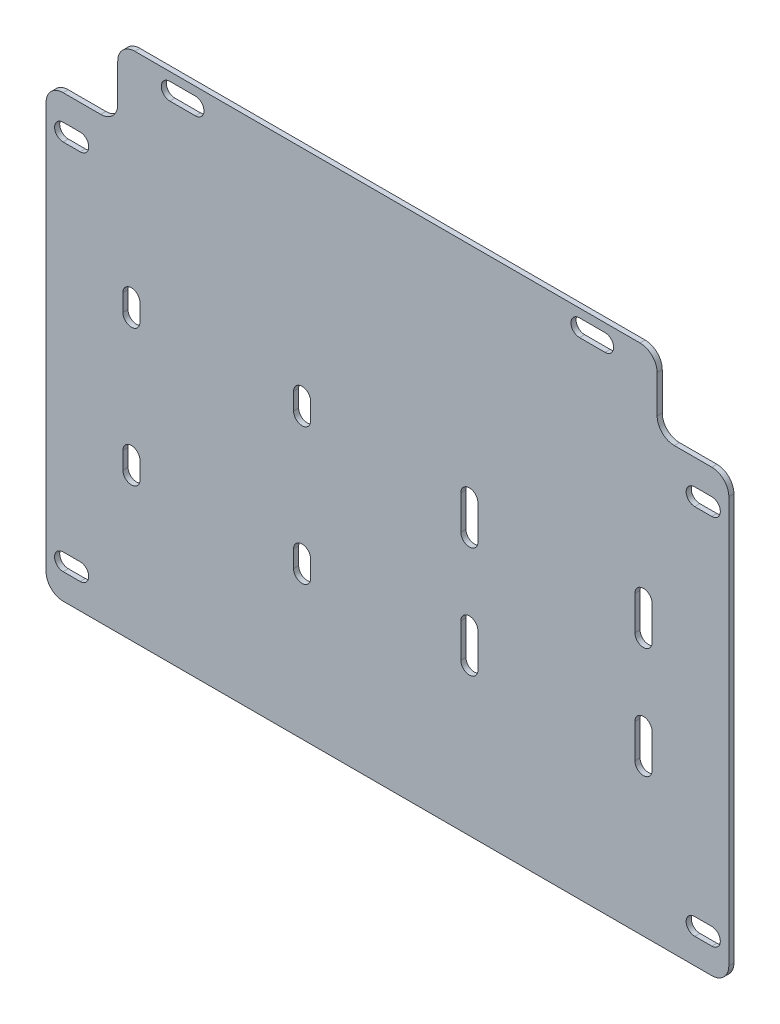
SolidWorks part; units mm, degrees
ref_plane "Front Plane" through (0, 0, 0) normal (0, 0, 1) x (1, 0, 0)
ref_plane "Top Plane" through (0, 0, 0) normal (0, 1, 0) x (1, 0, 0)
ref_plane "Right Plane" through (0, 0, 0) normal (1, 0, 0) x (0, 0, -1)
other "Configuration Table"
sketch "Sketch1" plane through (0, 0, 0) normal (0, 0, 1) x (1, 0, 0)
  line L0 (248, -128.5) -> (248, -148.5) construction
  line L1 (0, 0) -> (400, 0)
  line L2 (0, 0) -> (0, -342)
  line L3 (0, -342) -> (400, -342)
  line L4 (400, 0) -> (400, -342)
  line L5 (253, -128.5) -> (253, -148.5)
  line L6 (243, -128.5) -> (243, -148.5)
  line L7 (200, 0) -> (200, -342) construction
  line L8 (0, -171) -> (400, -171) construction
  line L9 (350, -128.5) -> (350, -148.5) construction
  line L10 (345, -128.5) -> (345, -148.5)
  line L11 (355, -128.5) -> (355, -148.5)
  line L12 (350, -213.5) -> (350, -193.5) construction
  line L13 (345, -213.5) -> (345, -193.5)
  line L14 (355, -213.5) -> (355, -193.5)
  line L15 (248, -213.5) -> (248, -193.5) construction
  line L16 (253, -213.5) -> (253, -193.5)
  line L17 (243, -213.5) -> (243, -193.5)
  line L18 (72.5, -10) -> (87.5, -10) construction
  line L19 (72.5, -5) -> (87.5, -5)
  line L20 (72.5, -15) -> (87.5, -15)
  line L21 (327.5, -10) -> (312.5, -10) construction
  line L22 (327.5, -5) -> (312.5, -5)
  line L23 (327.5, -15) -> (312.5, -15)
  line L24 (327.5, -332) -> (312.5, -332) construction
  line L25 (327.5, -337) -> (312.5, -337)
  line L26 (327.5, -327) -> (312.5, -327)
  line L27 (72.5, -332) -> (87.5, -332) construction
  line L28 (72.5, -337) -> (87.5, -337)
  line L29 (72.5, -327) -> (87.5, -327)
  line L30 (50, -126) -> (50, -136) construction
  line L31 (55, -126) -> (55, -136)
  line L32 (45, -126) -> (45, -136)
  line L33 (150, -126) -> (150, -136) construction
  line L36 (155, -126) -> (155, -136)
  line L37 (145, -126) -> (145, -136)
  line L38 (150, -216) -> (150, -206) construction
  line L39 (155, -216) -> (155, -206)
  line L40 (145, -216) -> (145, -206)
  line L41 (50, -216) -> (50, -206) construction
  line L42 (55, -216) -> (55, -206)
  line L43 (45, -216) -> (45, -206)
  arc A0 (253, -128.5) -> (243, -128.5) centre (248, -128.5) ccw
  arc A1 (243, -148.5) -> (253, -148.5) centre (248, -148.5) ccw
  arc A2 (345, -128.5) -> (355, -128.5) centre (350, -128.5) cw
  arc A3 (355, -148.5) -> (345, -148.5) centre (350, -148.5) cw
  arc A4 (345, -213.5) -> (355, -213.5) centre (350, -213.5) ccw
  arc A5 (355, -193.5) -> (345, -193.5) centre (350, -193.5) ccw
  arc A6 (253, -213.5) -> (243, -213.5) centre (248, -213.5) cw
  arc A7 (243, -193.5) -> (253, -193.5) centre (248, -193.5) cw
  arc A8 (72.5, -5) -> (72.5, -15) centre (72.5, -10) ccw
  arc A9 (87.5, -15) -> (87.5, -5) centre (87.5, -10) ccw
  arc A10 (327.5, -5) -> (327.5, -15) centre (327.5, -10) cw
  arc A11 (312.5, -15) -> (312.5, -5) centre (312.5, -10) cw
  arc A12 (327.5, -337) -> (327.5, -327) centre (327.5, -332) ccw
  arc A13 (312.5, -327) -> (312.5, -337) centre (312.5, -332) ccw
  arc A14 (72.5, -337) -> (72.5, -327) centre (72.5, -332) cw
  arc A15 (87.5, -327) -> (87.5, -337) centre (87.5, -332) cw
  arc A16 (55, -126) -> (45, -126) centre (50, -126) ccw
  arc A17 (45, -136) -> (55, -136) centre (50, -136) ccw
  arc A20 (155, -126) -> (145, -126) centre (150, -126) ccw
  arc A21 (145, -136) -> (155, -136) centre (150, -136) ccw
  arc A22 (155, -216) -> (145, -216) centre (150, -216) cw
  arc A23 (145, -206) -> (155, -206) centre (150, -206) cw
  arc A24 (55, -216) -> (45, -216) centre (50, -216) cw
  arc A25 (45, -206) -> (55, -206) centre (50, -206) cw
  point P7 (248, -138.5)
  point P18 (350, -138.5)
  point P25 (350, -203.5)
  point P32 (248, -203.5)
  point P39 (80, -10)
  point P46 (320, -10)
  point P53 (320, -332)
  point P60 (80, -332)
  point P67 (50, -131)
  point P74 (150, -131)
  point P81 (150, -211)
  point P88 (50, -211)
  dimension "D1" = 342
  dimension "D2" = 400
  dimension "D3" = 10
  dimension "D4" = 102
  dimension "D5" = 65
  dimension "D6" = 20
  dimension "D7" = 10
  dimension "D8" = 15
  dimension "D9" = 80
  dimension "D10" = 10
  dimension "D11" = 50
  dimension "D12" = 10
  dimension "D13" = 10
  dimension "D14" = 100
  dimension "D15" = 80
  dimension "D16" = 50
extrude "Boss-Extrude1" add sketch "Sketch1" along normal blind 3
sketch "Sketch3" plane through (0, 0, 3) normal (0, 0, 1) x (1, 0, 0)
  line L0 (200, 0) -> (200, -342) construction
  line L5 (400, 0) -> (0, 0) construction
  line L6 (0, -342) -> (400, -342) construction
  line L12 (0, 0) -> (0, -342) construction
  line L13 (-44.4488, -300) -> (42, -300)
  line L14 (-44.4488, -300) -> (-44.4488, -826.1424)
  line L15 (-44.4488, -826.1424) -> (42, -826.1424)
  line L16 (42, -300) -> (42, -826.1424)
  line L17 (0, -171) -> (400, -171) construction
  line L18 (400, -342) -> (400, 0) construction
  line L19 (444.4488, -826.1424) -> (358, -826.1424)
  line L20 (358, -300) -> (358, -826.1424)
  line L21 (444.4488, -300) -> (358, -300)
  line L22 (444.4488, -300) -> (444.4488, -826.1424)
  line L23 (444.4488, -42) -> (444.4488, 484.1424)
  line L24 (444.4488, -42) -> (358, -42)
  line L25 (358, -42) -> (358, 484.1424)
  line L26 (444.4488, 484.1424) -> (358, 484.1424)
  line L27 (-44.4488, 484.1424) -> (42, 484.1424)
  line L28 (42, -42) -> (42, 484.1424)
  line L29 (-44.4488, -42) -> (42, -42)
  line L30 (-44.4488, -42) -> (-44.4488, 484.1424)
  dimension "D1" = 42
  dimension "D2" = 42
extrude "Cut-Extrude2" cut sketch "Sketch3" against normal through all
fillet "Fillet1" radius 10 12 edges at (42, -42, 1.5) (42, 0, 1.5) (0, -42, 1.5) (358, 0, 1.5) (400, -42, 1.5) (358, -42, 1.5) (358, -342, 1.5) (358, -300, 1.5) (400, -300, 1.5) (0, -300, 1.5) (42, -300, 1.5) (42, -342, 1.5)
sketch "Sketch4" plane through (0, 0, 3) normal (0, 0, 1) x (1, 0, 0)
  line L0 (10, -62) -> (20, -62) construction
  line L1 (10, -57) -> (20, -57)
  line L2 (10, -67) -> (20, -67)
  line L3 (200, 0) -> (200, -342) construction
  line L4 (348, 0) -> (52, 0) construction
  line L5 (52, -342) -> (348, -342) construction
  line L6 (0, -171) -> (400, -171) construction
  line L7 (0, -52) -> (0, -290) construction
  line L8 (400, -290) -> (400, -52) construction
  line L9 (390, -62) -> (380, -62) construction
  line L10 (390, -57) -> (380, -57)
  line L11 (390, -67) -> (380, -67)
  line L12 (390, -280) -> (380, -280) construction
  line L13 (390, -285) -> (380, -285)
  line L14 (390, -275) -> (380, -275)
  line L15 (10, -280) -> (20, -280) construction
  line L16 (10, -285) -> (20, -285)
  line L17 (10, -275) -> (20, -275)
  line L18 (10, -42) -> (32, -42) construction
  arc A0 (10, -57) -> (10, -67) centre (10, -62) ccw
  arc A1 (20, -67) -> (20, -57) centre (20, -62) ccw
  arc A2 (390, -57) -> (390, -67) centre (390, -62) cw
  arc A3 (380, -67) -> (380, -57) centre (380, -62) cw
  arc A4 (390, -285) -> (390, -275) centre (390, -280) ccw
  arc A5 (380, -275) -> (380, -285) centre (380, -280) ccw
  arc A6 (10, -285) -> (10, -275) centre (10, -280) cw
  arc A7 (20, -275) -> (20, -285) centre (20, -280) cw
  point P2 (15, -62)
  point P21 (385, -62)
  point P28 (385, -280)
  point P35 (15, -280)
  dimension "D1" = 10
  dimension "D2" = 10
  dimension "D3" = 20
  dimension "D4" = 15
extrude "Cut-Extrude3" cut sketch "Sketch4" against normal through all
sketch "Sketch5" plane through (0, 0, 3) normal (0, 0, 1) x (1, 0, 0)
  line L5 (32, -300) -> (368, -300)
  line L6 (32, -300) -> (32, -515.5708)
  line L7 (32, -515.5708) -> (368, -515.5708)
  line L8 (368, -300) -> (368, -515.5708)
extrude "Cut-Extrude4" cut sketch "Sketch5" against normal blind 10
